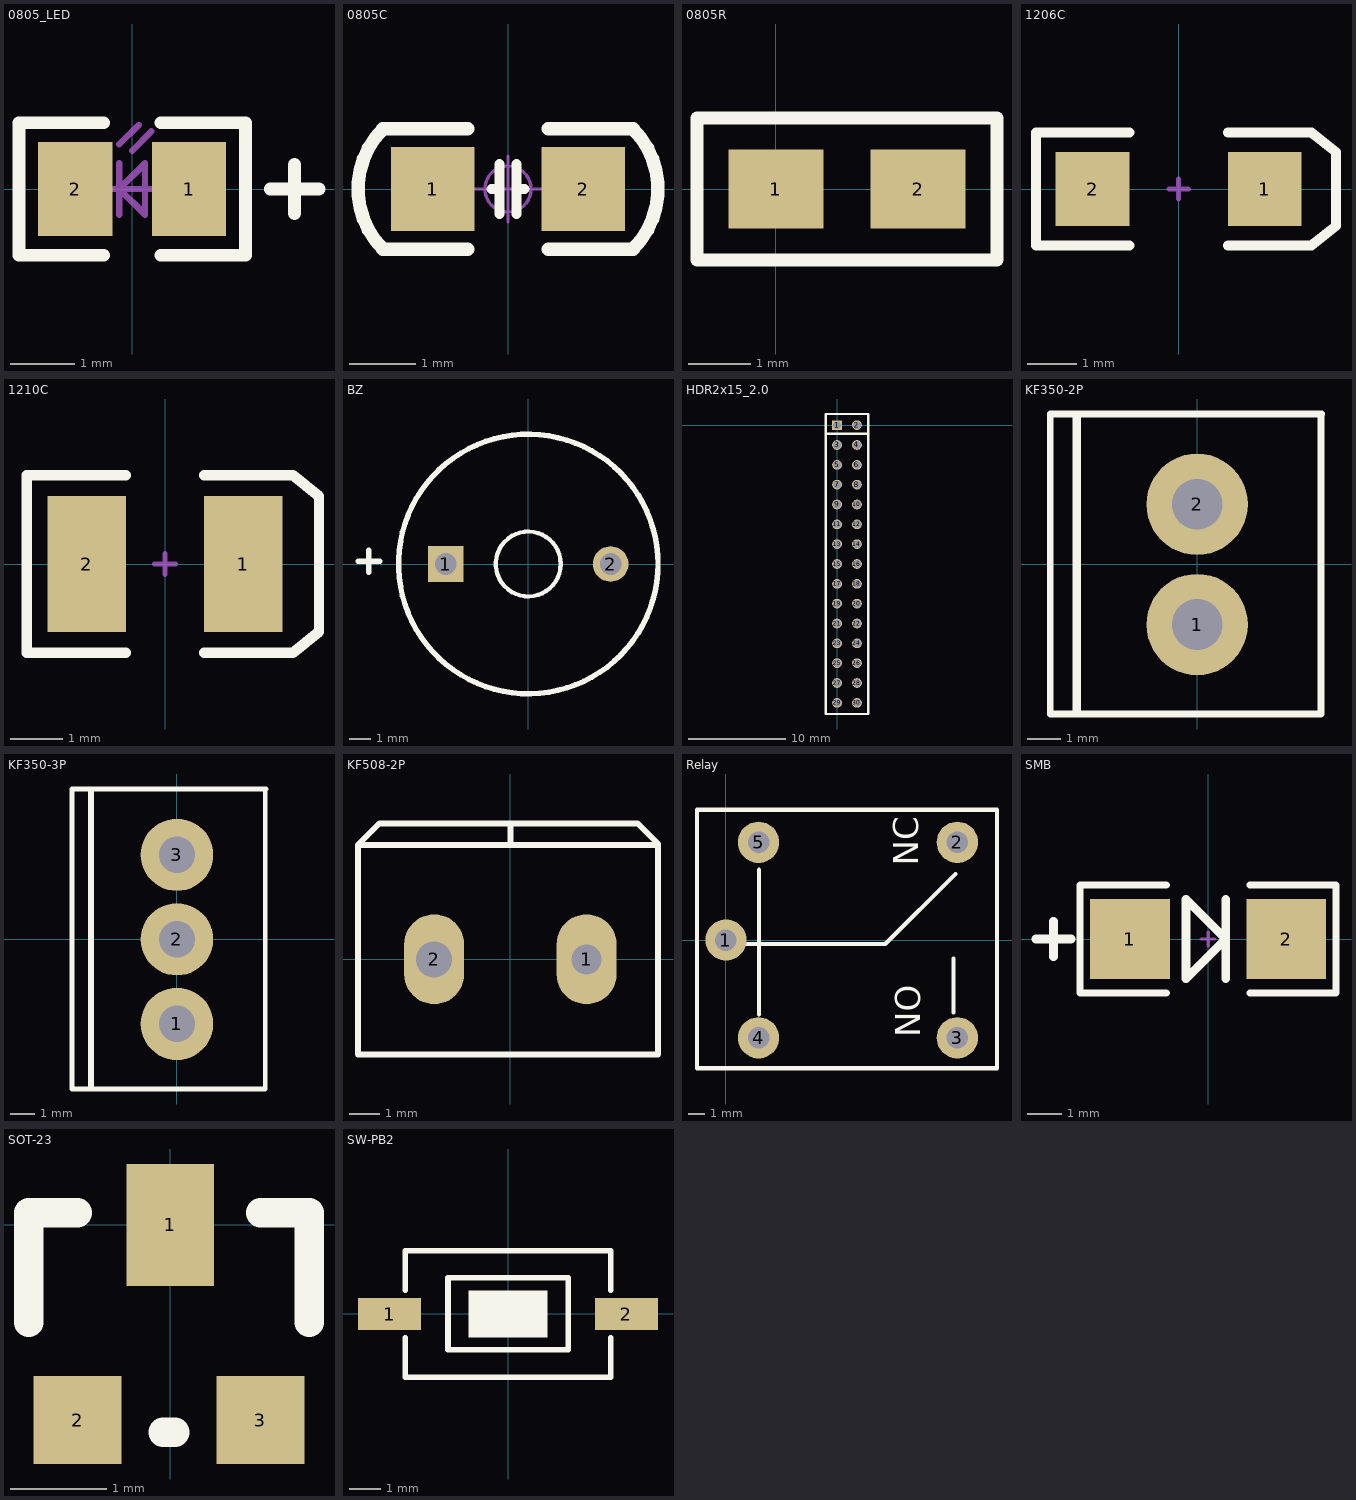
[diagram p0: the footprints below, top view; thin cyan lines are the x and y axes]
# Altium footprint library MISC82341-29.PcbLib: 14 footprints
Each footprint in its own frame and in the unit in brackets; x right, y up, seen from the top. Pads: shape width x height; smd on the part's side, far side on the other; paste and mask are expansions set on the pad; w line width, h text height; cw(c..) or ccw(c..) is an arc to the next point about the centre after c.

## 0805_LED [mm]
pads (2):
  rect 1.16x1.47 smd: 1(0.89,0) 2(-0.89,0)
Top Overlay:
  lines w0.2: -0.45,-1.035 -1.77,-1.035 -1.77,1.035 -0.45,1.035 ; 0.45,-1.035 1.77,-1.035 1.77,1.035 0.45,1.035 ; 2.159,0 2.921,0 ; 2.54,-0.381 2.54,0.381
Mechanical 13:
  lines w0.1: -0.4,0 0.4,0 ; -0.2,-0.4 -0.2,0.4 ; -0.2,0.7 0.1,1 ; 0,0.6 0.3,0.9 ; -0.2,0 0.2,0.4 0.2,-0.4 -0.2,0
3D body "User Library-led_0805.step": height 1.1, standoff 0, extent -1.01,-0.625 1.01,0.625

## 0805C [mil] "Non-polar chip capacitor"
height 19.68
pads (2):
  rect 50x50 smd: 1(-45,0) 2(45,0)
Top Overlay:
  lines w6: -10,0 -5,0 ; -5,-15 -5,15 ; 5,-15 5,15 ; 5,0 10,0
  lines w7.99: -74.8,-36 cw(c-38.8,0) -74.8,36 ; 74.8,-36 ccw(c38.8,0) 74.8,36
  lines w8: -74.8,-36 -24,-36 ; -74.8,36 -24,36 ; 24,-36 74.8,-36 ; 24,36 74.8,36
Mechanical 15:
  circle w1.97: c0,0 r13.78
  lines w1.97: -19.69,0 19.68,0 ; 0,-19.68 0,19.69
3D body "C 0805.STEP": height 20.08, standoff -0.39, extent -39.37,-24.02 39.37,24.02

## 0805R [mil]
pads (2):
  rect 60x50 smd: 1(0,0) 2(90,0)
Top Overlay:
  lines w8: -50,-45 -50,45 65,45 140,45 140,-45 65,-45 -50,-45
3D body "R0805.STEP": height 21.65, standoff 0, extent 4.64,-24.8 83.37,24.81

## 1206C [mm] "SMT LED; 2 Flat Leads"
height 1.2
pads (2):
  rect 1.5x1.5 smd: 1(1.75,0) 2(-1.75,0)
Top Overlay:
  lines w0.2: -1,-1.15 -2.9,-1.15 -2.9,1.15 -1,1.15 ; 1,-1.15 2.7,-1.15 3.2,-0.75 3.2,0.75 2.7,1.15 1,1.15
Mechanical 1:
  lines w0.1: -0.2,0 0.2,0 ; 0,-0.2 0,0.2

## 1210C [mm] "SM LED; 2 C-Bend Leads; Body 3.5 x 2.8 x 1.9 mm, inc leads (LxWxH typ)"
height 1.9
pads (2):
  rect 1.5x2.6 smd: 1(1.5,0) 2(-1.5,0)
Top Overlay:
  lines w0.2: -0.75,-1.7 -2.65,-1.7 -2.65,1.7 -0.75,1.7 ; 0.75,-1.7 2.45,-1.7 2.95,-1.3 2.95,1.3 2.45,1.7 0.75,1.7
Mechanical 1:
  lines w0.1: -0.2,0 0.2,0 ; 0,-0.2 0,0.2

## BZ [mm]
pads (2):
  rect 1.65x1.65 hole 1: 1(-3.81,0)
  round 1.65 hole 1: 2(3.81,0)
Top Overlay:
  circle w0.2: c0,0 r1.5
  circle w0.254: c0,0 r6
  lines w0.254: -7.874,0.127 -6.858,0.127 ; -7.366,-0.381 -7.366,0.635

## HDR2x15_2.0 [mm]
pads (30):
  rect 1x1 hole 0.8: 1(0,0)
  round 1 hole 0.8: 2(2.032,0) 3(0,-2.032) 4(2.032,-2.032) 5(0,-4.064) 6(2.032,-4.064) 7(0,-6.096) 8(2.032,-6.096) 9(0,-8.128) 10(2.032,-8.128) 11(0,-10.16) 12(2.032,-10.16) 13(0,-12.192) 14(2.032,-12.192) 15(0,-14.224) 16(2.032,-14.224) 17(0,-16.256) 18(2.032,-16.256) 19(0,-18.288) 20(2.032,-18.288) 21(0,-20.32) 22(2.032,-20.32) 23(0,-22.352) 24(2.032,-22.352) 25(0,-24.384) 26(2.032,-24.384) 27(0,-26.416) 28(2.032,-26.416) 29(0,-28.448) 30(2.032,-28.448)
Top Overlay:
  lines w0.254: -1.016,-0.889 3.048,-0.889 ; -1.143,-29.591 -1.143,-29.337 -1.143,-0.762 -1.143,0.508 -1.143,1.143 3.175,1.143 3.175,0.508 3.175,-0.635 3.175,-29.591 -1.143,-29.591

## KF350-2P [mm]
pads (2):
  round 3 hole 1.5: 1(0,-1.778) 2(0,1.778)
Top Overlay:
  lines w0.2: -4.343,4.445 -4.343,-4.42 3.658,-4.42 3.658,4.445 ; -4.318,4.445 3.683,4.445
  lines w0.254: -3.556,-4.318 -3.556,4.318

## KF350-3P [mm]
pads (3):
  round 3 hole 1.5: 1(0,-3.5) 2(0,0) 3(0,3.5)
Top Overlay:
  lines w0.2: -4.343,6.223 -4.343,-6.198 3.658,-6.198 3.658,6.223 ; -4.318,6.223 3.683,6.223
  lines w0.254: -3.556,-6.096 -3.556,6.096

## KF508-2P [mm]
height 10
pads (2):
  oval 2x3 hole 1: 1(2.54,0)
  oval 2x3 hole 1.2: 2(-2.54,0)
Top Overlay:
  lines w0.203: 0,3.81 0,4.445 ; 4.887,3.81 -5.08,3.81 ; -5.08,3.81 -5.08,-3.175 4.92,-3.175 4.92,3.843 4.238,4.525 -4.365,4.525 -5.08,3.81
3D body "User Library-Terminal block 2 POS.STEP": height 10, standoff -3.05, extent -5.156,-3.173 5.004,4.327

## Relay [mm]
pads (5):
  round 2.54 hole 1.321: 1(0,0) 2(14.2,6) 3(14.2,-6) 4(2,-6) 5(2,6)
Top Overlay:
  lines w0.254: 1.27,-0.254 9.779,-0.254 14.097,4.064 ; 2.032,-4.572 2.032,4.318 ; 13.97,-4.445 13.97,-1.143 ; -1.778,-7.874 16.637,-7.874 16.637,8.001 -1.778,8.001 -1.778,-7.747 -1.778,-7.874
  text "NC" at 11.811,4.572 h1.52
  text "NO" at 11.938,-5.969 h1.52

## SMB [mm] "DO-214-AA/SMB; 2 C-Bend Leads; Body 5.3 x 3.6 mm, inc. leads (LxW)"
height 2.54
pads (2):
  rect 2.3x2.3 smd: 1(-2.25,0) 2(2.25,0)
Top Overlay:
  lines w0.2: -1.2,-1.55 -3.683,-1.55 -3.683,1.55 -1.2,1.55 ; 1.2,-1.55 3.683,-1.55 3.683,1.55 1.2,1.55
  lines w0.254: -4.953,0 -4.191,0 -3.937,0 ; -4.445,-0.508 -4.445,0.508 ; 0.508,-1.143 0.508,1.143 ; -0.635,-1.143 0.508,0 -0.635,1.143 -0.635,0.635 -0.635,-0.762 -0.635,-1.143
Mechanical 1:
  lines w0.1: -0.2,0 0.2,0 ; 0,-0.2 0,0.2

## SOT-23 [mil]
pads (3):
  rect 36x50 smd: 1(0,0)
  rect 36x36 smd: 2(-38,-80) 3(37,-80)
Top Overlay:
  lines w12: -58,-40 -58,5 -38,5 ; -3,-85 2,-85 ; 37,5 57,5 57,-40

## SW-PB2 [mm]
pads (2):
  rect 2x1 smd: 1(-3.756,-0.008) 2(3.744,-0.008)
Top Overlay:
  rectangle: -1.256,-0.757 1.244,0.742
  lines w0.178: -3.256,-0.757 -3.256,-2.008 3.244,-2.008 3.244,-0.757 ; -3.256,0.742 -3.256,1.993 3.244,1.993 3.244,0.742 ; -1.905,-1.143 -1.905,1.143 1.905,1.143 1.905,-1.143 -1.905,-1.143